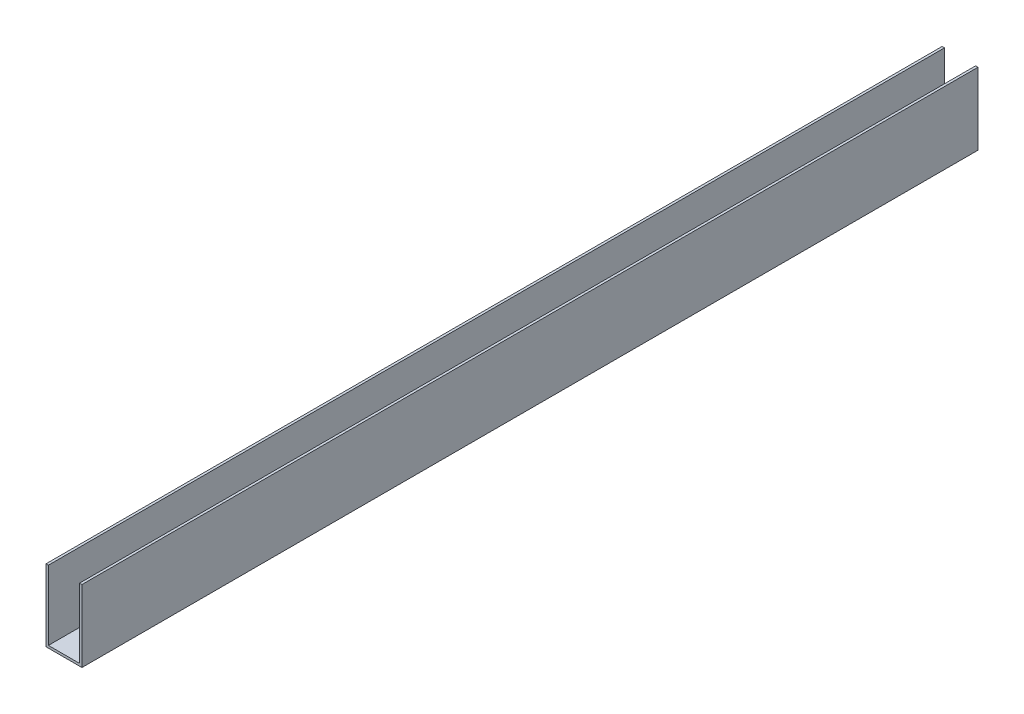
from build123d import *

# Parameters (mm, degrees)
SKETCH_1_W      = 30
SKETCH_1_H      = 60
EXTRUDE_1_DEPTH = 374
SHELL_1_T       = -2


with BuildPart() as part:
    # 草图1 → 凸台-拉伸1 (new, symmetric)
    with BuildSketch(Plane.XY):
        Rectangle(SKETCH_1_W, SKETCH_1_H)
    extrude(amount=EXTRUDE_1_DEPTH, both=True)

    # 抽壳1
    shell_1_openings = [part.faces().sort_by_distance(p)[0] for p in [
        (0, 0, 374),
        (0, 0, -374),
        (0, 30, 0),
    ]]
    offset(amount=SHELL_1_T, openings=shell_1_openings, kind=Kind.INTERSECTION)


solid = part.part
